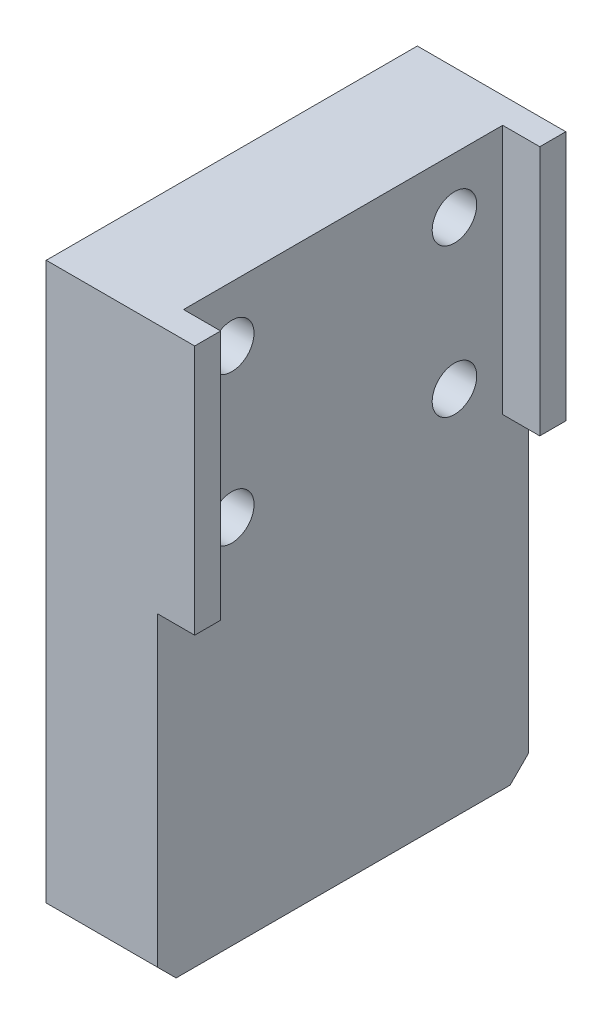
SolidWorks part; units mm, degrees
material "AL6061"
ref_plane "Front Plane" through (0, 0, 0) normal (0, 0, 1) x (1, 0, 0)
ref_plane "Top Plane" through (0, 0, 0) normal (0, 1, 0) x (1, 0, 0)
ref_plane "Right Plane" through (0, 0, 0) normal (1, 0, 0) x (0, 0, -1)
sketch "Sketch2" plane through (0, 0, 0) normal (1, 0, 0) x (0, 0, -1)
  line L1 (-10, -15.5) -> (10, -15.5)
  line L2 (-10, -15.5) -> (-10, 15.5)
  line L3 (-10, 15.5) -> (10, 15.5)
  line L4 (10, -15.5) -> (10, 15.5)
  line L5 (-10, -15.5) -> (10, 15.5) construction
  line L6 (-10, 15.5) -> (10, -15.5) construction
  point P0 (0, 0)
  dimension "D1" = 20
  dimension "D2" = 31
extrude "Boss-Extrude1" add sketch "Sketch2" along normal blind 6
sketch "Sketch3" plane through (6, 0, 0) normal (1, 0, 0) x (0, 0, -1)
  line L0 (-10, -15.5) -> (10, -15.5) construction
  line L1 (-10, 15.5) -> (-8.6, 15.5)
  line L2 (-10, 15.5) -> (-10, -15.5)
  line L3 (-10, -15.5) -> (-8.6, -15.5)
  line L4 (-8.6, 15.5) -> (-8.6, -15.5)
  line L5 (0, 0) -> (0, 15.5) construction
  line L6 (10, 15.5) -> (-10, 15.5) construction
  line L7 (8.6, 15.5) -> (8.6, -15.5)
  line L8 (10, -15.5) -> (8.6, -15.5)
  line L9 (10, 15.5) -> (10, -15.5)
  line L10 (10, 15.5) -> (8.6, 15.5)
  dimension "D1" = 17.2
extrude "Boss-Extrude2" add sketch "Sketch3" along normal blind 2
sketch "Sketch4" plane through (0, 0, 10) normal (0, 0, 1) x (1, 0, 0)
  line L0 (8, 15.5) -> (0, 15.5) construction
  line L1 (8, -15.5) -> (6, -15.5)
  line L2 (8, -15.5) -> (8, 2)
  line L3 (8, 2) -> (6, 2)
  line L4 (6, -15.5) -> (6, 2)
  dimension "D1" = 2
  dimension "D2" = 13.5
extrude "Cut-Extrude1" cut sketch "Sketch4" against normal through all
hole_wizard "CBORE for M2 Hexagon socket head cap screws1" positions "Sketch5" profile "Sketch6" counterbore size "M2" standard "GB"
sketch "Sketch5" plane through (0, 0, 0) normal (-1, 0, 0) x (0, 0, 1)
  line L3 (0, 15.5) -> (0, 2) construction
  line L4 (-8.6, 15.5) -> (8.6, 15.5) construction
  line L9 (-10, 15.5) -> (10, 15.5) construction
  point P0 (6, 12.5)
  point P2 (-6, 12.5)
  point P4 (-6, 4.5)
  point P6 (6, 4.5)
  dimension "D1" = 12
  dimension "D2" = 8
  dimension "D3" = 3
sketch "Sketch6" plane through (0, 12.5, 6) normal (0, 1, 0) x (0, 0, 1)
  line L0 (0, 0) -> (0, 10.821)
  line L1 (0, 10.821) -> (1.2, 10.1)
  line L2 (1.2, 10.1) -> (1.2, 2.3)
  line L3 (1.2, 2.3) -> (2.15, 2.3)
  line L4 (2.15, 2.3) -> (2.15, 0)
  line L5 (2.15, 0) -> (0, 0)
  line L10 (0, 10.821) -> (-1.2, 10.1) construction
  line L11 (0, -6.35) -> (0, 107.95) construction
  dimension "孔直径" = 2.4
  dimension "孔深度" = 10.1
  dimension "柱形沉头孔直径" = 4.3
  dimension "柱形沉头孔深度" = 2.3
  dimension "导头角度" = 118
hole_wizard "M3 Tapped Hole1" positions "Sketch10" profile "Sketch11" tap size "M3" standard "GB"
sketch "Sketch10" plane through (0, -15.5, 0) normal (0, -1, 0) x (-1, 0, 0)
  line L0 (-3, 10) -> (-3, 0) construction
  line L1 (-6, 10) -> (0, 10) construction
  line L2 (-3, 0) -> (0, 0) construction
  point P0 (-3, 5)
  point P2 (-3, -5)
  dimension "D1" = 10
sketch "Sketch11" plane through (3, -15.5, -5) normal (1, 0, 0) x (0, 0, -1)
  line L0 (0, 0) -> (0, 8.2511)
  line L1 (0, 8.2511) -> (1.25, 7.5)
  line L2 (1.25, 7.5) -> (1.25, 0)
  line L5 (1.25, 0) -> (0, 0)
  line L10 (0, 8.2511) -> (-1.25, 7.5) construction
  line L11 (0, -6.35) -> (0, 107.95) construction
  dimension "螺纹孔钻头直径" = 2.5
  dimension "螺纹孔钻头深度" = 7.5
  dimension "导头角度" = 118
cosmetic thread "Cosmetic Thread 1" parameters "D1"=6, "D2"=3
cosmetic thread "Cosmetic Thread 2" parameters "D1"=6, "D2"=3
chamfer "Chamfer1" distance 1 angle 45 2 edges at (3, -15.5, 10) (3, -15.5, -10)
